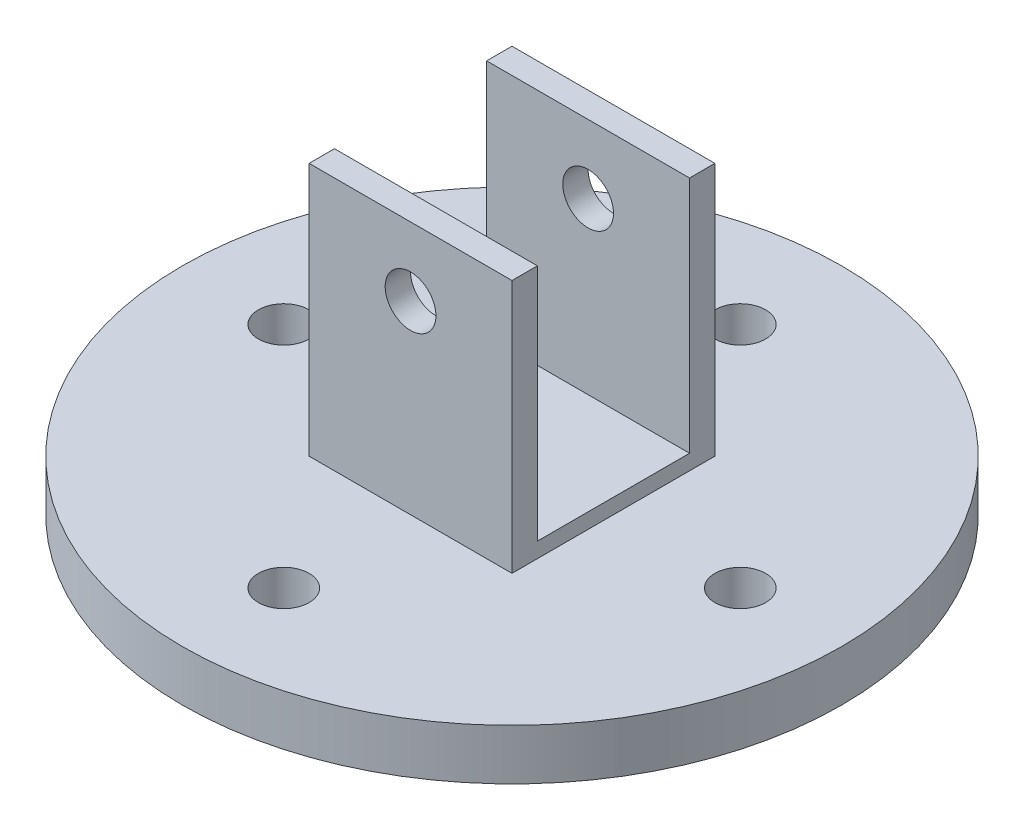
SolidWorks part; units mm, degrees
ref_plane "Front Plane" through (0, 0, 0) normal (0, 0, 1) x (1, 0, 0)
ref_plane "Top Plane" through (0, 0, 0) normal (0, 1, 0) x (1, 0, 0)
ref_plane "Right Plane" through (0, 0, 0) normal (1, 0, 0) x (0, 0, -1)
other "Configuration Table"
sketch "Sketch1" plane through (0, 0, 0) normal (0, 1, 0) x (1, 0, 0)
  circle A0 centre (0, 0) radius 65
  circle A1 centre (0, 0) radius 15
  dimension "D1" = 130
  dimension "D2" = 30
extrude "Boss-Extrude1" add sketch "Sketch1" along normal blind 10
sketch "Sketch2" plane through (0, 10, 0) normal (0, 1, 0) x (1, 0, 0)
  line L0 (0, 0) -> (0, -50000) construction
  line L1 (0, 0) -> (50000, 0) construction
  circle A0 centre (0, 0) radius 45 construction
  circle A1 centre (0, 45) radius 5
  circle A2 centre (45, 0) radius 5
  circle A3 centre (0, -45) radius 5
  circle A4 centre (-45, 0) radius 5
  dimension "D1" = 90
  dimension "D2" = 10
extrude "Cut-Extrude1" cut sketch "Sketch2" against normal blind 10
sketch "Sketch3" plane through (0, 10, 0) normal (0, 1, 0) x (1, 0, 0)
  line L1 (-20, -20) -> (20, -20)
  line L2 (-20, -20) -> (-20, 20)
  line L3 (-20, 20) -> (20, 20)
  line L4 (20, -20) -> (20, 20)
  line L5 (0, 20) -> (0, -20) construction
  line L6 (-20, 0) -> (20, 0) construction
  point P0 (0, 0)
  dimension "D1" = 40
  dimension "D2" = 40
extrude "Boss-Extrude2" add sketch "Sketch3" along normal blind 50
sketch "Sketch4" plane through (20, 0, 0) normal (1, 0, 0) x (0, 0, -1)
  line L0 (0, 0) -> (0, 50000) construction
  line L1 (-20, 60) -> (20, 60) construction
  line L2 (-15, 60) -> (15, 60)
  line L3 (-15, 60) -> (-15, 13)
  line L4 (-15, 13) -> (15, 13)
  line L5 (15, 60) -> (15, 13)
  line L6 (-20, 10) -> (20, 10) construction
  dimension "D1" = 30
  dimension "D2" = 15
  dimension "D3" = 3
extrude "Cut-Extrude2" cut sketch "Sketch4" against normal blind 50
sketch "Sketch5" plane through (0, 0, 20) normal (0, 0, 1) x (1, 0, 0)
  line L0 (0, 0) -> (0, 50000) construction
  circle A0 centre (0, 46.4691) radius 5
  dimension "D1" = 10
extrude "Cut-Extrude3" cut sketch "Sketch5" against normal through all
